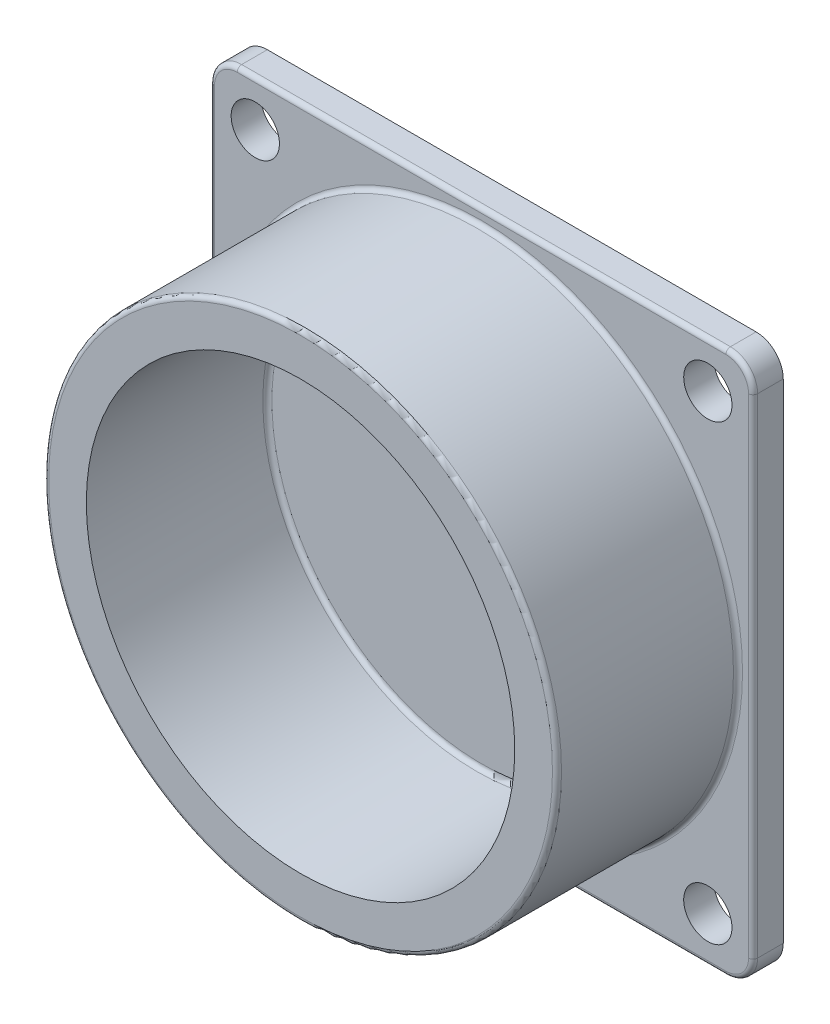
SolidWorks part; units mm, degrees
material "6061 Alloy"
ref_plane "Front Plane" through (0, 0, 0) normal (0, 0, 1) x (1, 0, 0)
ref_plane "Top Plane" through (0, 0, 0) normal (0, 1, 0) x (1, 0, 0)
ref_plane "Right Plane" through (0, 0, 0) normal (1, 0, 0) x (0, 0, -1)
sketch "Sketch1" plane through (0, 0, 0) normal (0, 0, 1) x (1, 0, 0)
  line L0 (0, 90) -> (0, 0) construction
  line L1 (-81, -90) -> (81, -90)
  line L2 (-90, -81) -> (-90, 81)
  line L3 (-81, 90) -> (81, 90)
  line L4 (90, -81) -> (90, 81)
  line L5 (-90, -90) -> (90, 90) construction
  line L6 (-90, 90) -> (90, -90) construction
  line L7 (0, 0) -> (90, 0) construction
  arc A0 (81, -90) -> (90, -81) centre (81, -81) ccw
  arc A1 (-81, -90) -> (-90, -81) centre (-81, -81) cw
  arc A2 (81, 90) -> (90, 81) centre (81, 81) cw
  arc A3 (-90, 81) -> (-81, 90) centre (-81, 81) cw
  circle A4 centre (0, 0) radius 9
  circle A5 centre (70, 70) radius 4.5
  circle A6 centre (-70, 70) radius 4.5
  circle A7 centre (70, -70) radius 4.5
  circle A8 centre (-70, -70) radius 4.5
  point P0 (0, 0)
  dimension "D2" = 9
  dimension "D3" = 18
  dimension "D4" = 9
  dimension "D1" = 180
  dimension "D5" = 70
extrude "Boss-Extrude1" add sketch "Sketch1" along normal blind 10
sketch "Sketch2" plane through (0, 0, 10) normal (0, 0, 1) x (1, 0, 0)
  circle A0 centre (0, 0) radius 85
  dimension "D1" = 170
extrude "Boss-Extrude2" add sketch "Sketch2" along normal blind 60
sketch "Sketch3" plane through (0, 0, 70) normal (0, 0, 1) x (1, 0, 0)
  circle A0 centre (0, 0) radius 71
  dimension "D1" = 142
extrude "Cut-Extrude1" cut sketch "Sketch3" against normal blind 60
fillet "Fillet1" radius 1.5 11 edges at (87.364, -87.364, 10) (0, -90, 10) (-87.364, -87.364, 10) (-90, 0, 10) (-87.364, 87.364, 10) (0, 90, 10) (87.364, 87.364, 10) (90, 0, 10) (85, 0, 10) (85, 0, 70) (71, 0, 10)
scale "Scale1" bodies to scale 103 scale about origin uniform scaling yes scale factor 0.5
sketch "草图1" plane through (0, 0, 0) normal (0, 0, -1) x (-1, 0, 0)
  circle A0 centre (35, -35) radius 2.25 construction
  circle A1 centre (-35, -35) radius 2.25 construction
  circle A2 centre (-35, 35) radius 2.25 construction
  circle A3 centre (35, 35) radius 2.25 construction
  circle A4 centre (35, -35) radius 2.25
  circle A5 centre (-35, -35) radius 2.25
  circle A6 centre (-35, 35) radius 2.25
  circle A7 centre (35, 35) radius 2.25
extrude "凸台-拉伸1" add sketch "草图1" against normal up to surface (5 mm away) up to face at (0, 0, 5)
sketch "草图2" plane through (0, 0, 0) normal (0, 0, -1) x (-1, 0, 0)
  line L0 (0, 0) -> (0, 66.4295) construction
  line L1 (-37.5, 37.5) -> (37.5, 37.5) construction
  line L2 (-37.5, 37.5) -> (-37.5, -37.5) construction
  line L3 (-37.5, -37.5) -> (37.5, -37.5) construction
  line L4 (37.5, 37.5) -> (37.5, -37.5) construction
  line L5 (-37.5, 37.5) -> (37.5, -37.5) construction
  line L6 (-37.5, -37.5) -> (37.5, 37.5) construction
  line L7 (0, 0) -> (-64.5739, 0) construction
  circle A0 centre (-37.5, 37.5) radius 4
  circle A1 centre (-37.5, -37.5) radius 4
  circle A2 centre (37.5, 37.5) radius 4
  circle A3 centre (37.5, -37.5) radius 4
  point P0 (0, 0)
  dimension "D2" = 8
  dimension "D1" = 75
extrude "切除-拉伸1" cut sketch "草图2" against normal blind 10
